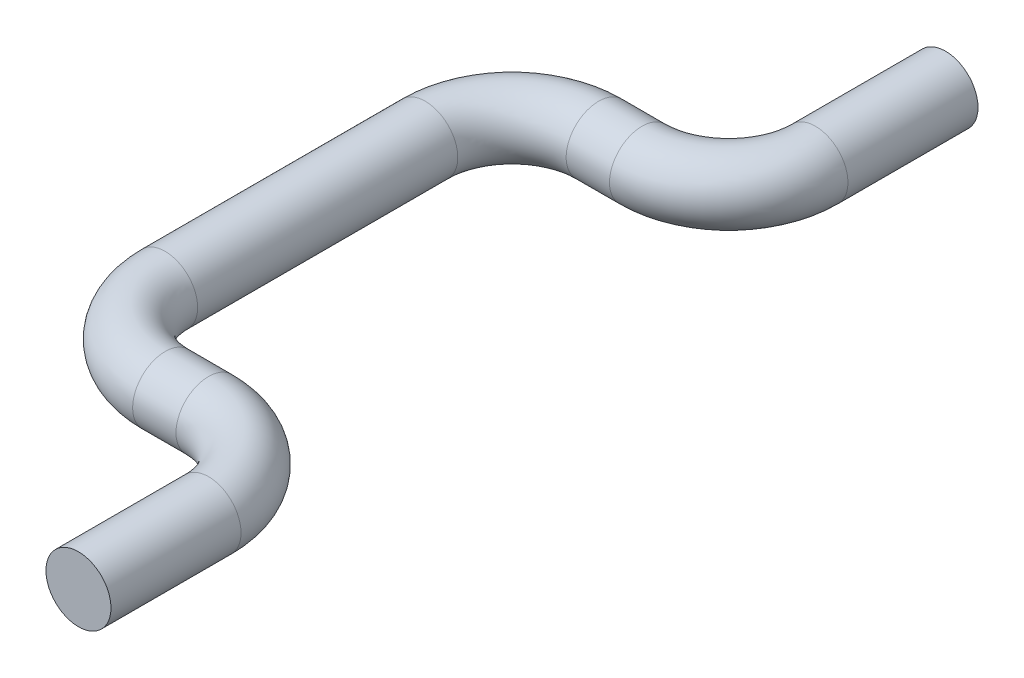
SolidWorks part; units mm, degrees
material "1023 碳钢板 (SS)"
ref_plane "Front Plane" through (0, 0, 0) normal (0, 0, 1) x (1, 0, 0)
ref_plane "Top Plane" through (0, 0, 0) normal (0, 1, 0) x (1, 0, 0)
ref_plane "Right Plane" through (0, 0, 0) normal (1, 0, 0) x (0, 0, -1)
sketch "Sketch1" plane through (0, 0, 0) normal (0, 1, 0) x (1, 0, 0)
  line L0 (0, 160) -> (0, 136)
  line L1 (-16, 120) -> (-24, 120)
  line L2 (-40, 104) -> (-40, 56)
  line L3 (-24, 40) -> (-16, 40)
  line L4 (0, 24) -> (0, 0)
  arc A0 (-40, 104) -> (-24, 120) centre (-24, 104) cw
  arc A1 (-24, 40) -> (-40, 56) centre (-24, 56) cw
  arc A2 (0, 136) -> (-16, 120) centre (-16, 136) cw
  arc A3 (0, 24) -> (-16, 40) centre (-16, 24) ccw
  point P9 (-40, 120)
  point P12 (-40, 40)
  point P15 (0, 120)
  dimension "D6" = 16
  dimension "D7" = 16
  dimension "D8" = 16
  dimension "D9" = 16
  dimension "D1" = 160
  dimension "D2" = 80
  dimension "D3" = 40
  dimension "D4" = 40
  dimension "D5" = 40
sketch "Sketch2" plane through (0, 0, 0) normal (0, 0, 1) x (1, 0, 0)
  circle A0 centre (0, 0) radius 6
  dimension "D1" = 12
sweep "Sweep1" add profiles "Sketch2" path "Sketch1"
